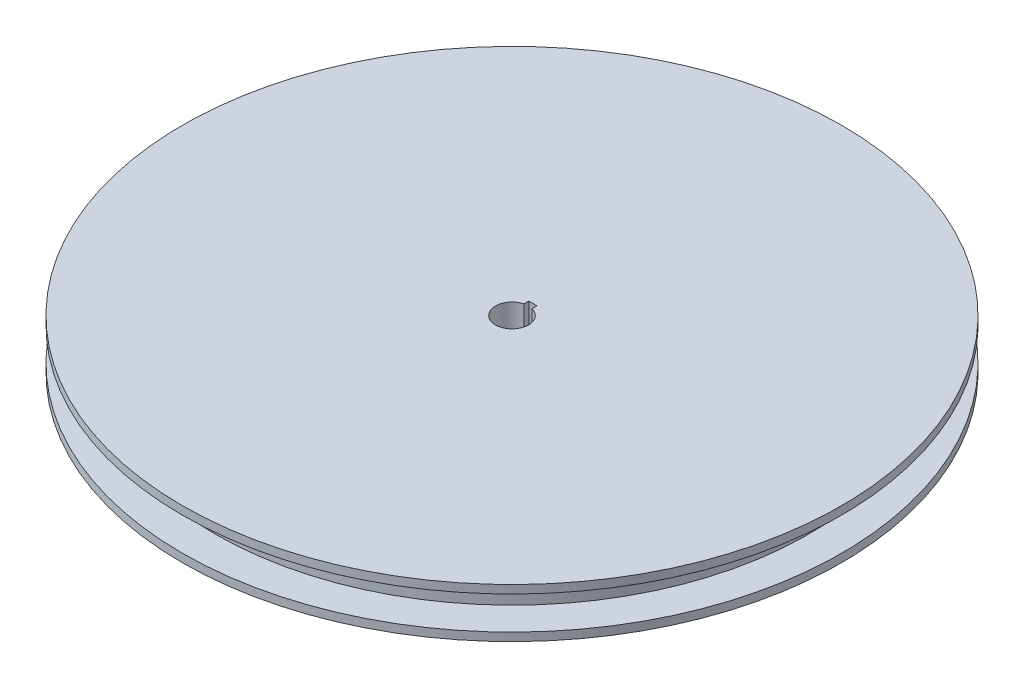
SolidWorks part; units mm, degrees
ref_plane "Front Plane" through (0, 0, 0) normal (0, 0, 1) x (1, 0, 0)
ref_plane "Top Plane" through (0, 0, 0) normal (0, 1, 0) x (1, 0, 0)
ref_plane "Right Plane" through (0, 0, 0) normal (1, 0, 0) x (0, 0, -1)
sketch "Sketch1" plane through (0, 0, 0) normal (0, 0, 1) x (1, 0, 0)
  line L0 (0, 76.7586) -> (0, -32.738) construction
  line L1 (-10, 0) -> (-10, -30)
  line L2 (-10, -30) -> (-200, -30)
  line L3 (-200, -30) -> (-200, -25)
  line L4 (-200, -25) -> (-180, -25)
  line L5 (-180, -25) -> (-180, -5)
  line L6 (-180, -5) -> (-200, -5)
  line L7 (-200, -5) -> (-200, 0)
  line L8 (-200, 0) -> (-10, 0)
  line L9 (0, 0) -> (-73.7995, 0) construction
  dimension "D1" = 10
  dimension "D2" = 200
  dimension "D3" = 180
  dimension "D4" = 5
  dimension "D5" = 20
revolve "Revolve1" add sketch "Sketch1" angle 360 about L0
sketch "Sketch2" plane through (0, 0, 0) normal (0, 1, 0) x (1, 0, 0)
  line L0 (0, 20.0252) -> (0, -7.5886) construction
  line L1 (-2.5, 12.6825) -> (-2.5, 9.6825)
  line L2 (-2.5, 12.6825) -> (2.5, 12.6825)
  line L3 (2.5, 12.6825) -> (2.5, 9.6825)
  circle A0 centre (0, 0) radius 10 construction
  arc A1 (2.5, 9.6825) -> (-2.5, 9.6825) centre (0, 0) ccw
  dimension "D1" = 3
  dimension "D2" = 5
extrude "Cut-Extrude1" cut sketch "Sketch2" against normal through all
